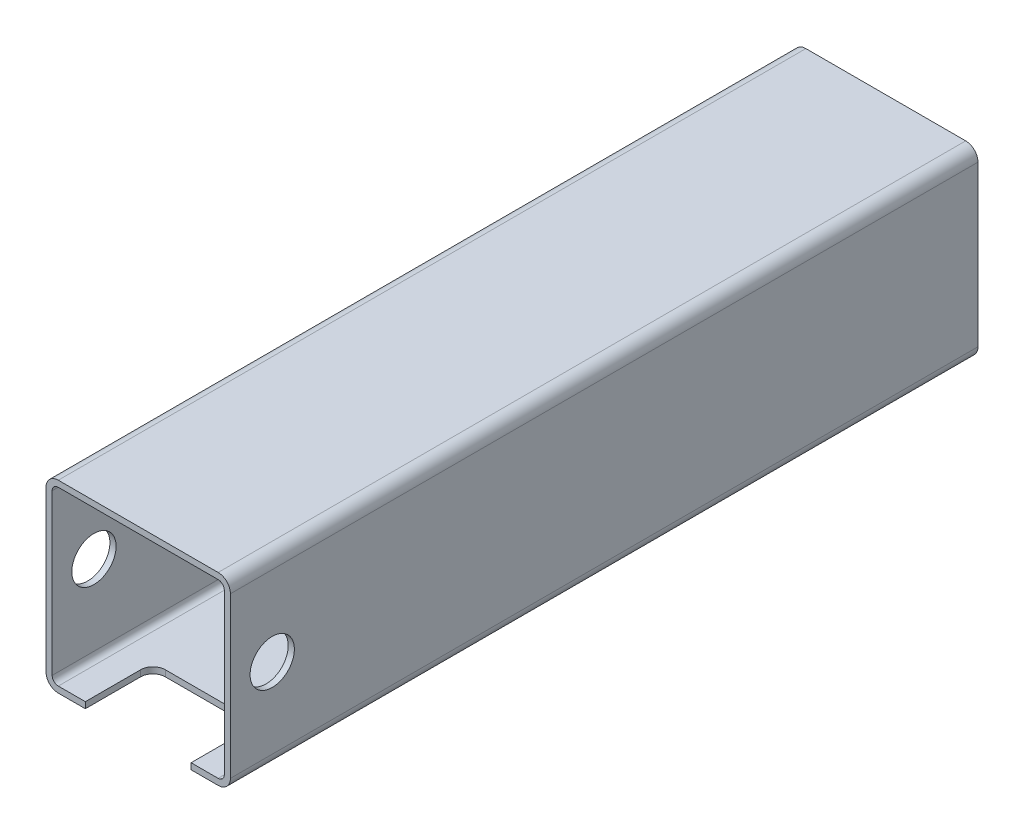
SolidWorks part; units mm, degrees
material "Q345"
ref_plane "Front Plane" through (0, 0, 0) normal (0, 0, 1) x (1, 0, 0)
ref_plane "Top Plane" through (0, 0, 0) normal (0, 1, 0) x (1, 0, 0)
ref_plane "Right Plane" through (0, 0, 0) normal (1, 0, 0) x (0, 0, -1)
sketch "Sketch1" plane through (0, 0, 0) normal (0, 0, 1) x (1, 0, 0)
  line L1 (0, 0) -> (150, 0)
  line L2 (0, 0) -> (0, 150)
  line L3 (0, 150) -> (150, 150)
  line L4 (150, 0) -> (150, 150)
  line L5 (5, 145) -> (145, 145)
  line L6 (5, 145) -> (5, 5)
  line L7 (5, 5) -> (145, 5)
  line L8 (145, 145) -> (145, 5)
  dimension "D1" = 150
  dimension "D2" = 150
  dimension "D3" = 5
  dimension "D4" = 5
  dimension "D5" = 5
  dimension "D6" = 5
extrude "Boss-Extrude1" add sketch "Sketch1" along normal blind 608
fillet "Fillet1" radius 10 4 edges at (150, 0, 304) (0, 0, 304) (0, 150, 304) (150, 150, 304)
fillet "Fillet2" radius 5 4 edges at (5, 5, 304) (145, 5, 304) (145, 145, 304) (5, 145, 304)
sketch "Sketch2" plane through (0, 0, 0) normal (-1, 0, 0) x (0, 0, 1)
  line L0 (0, 150) -> (608, 150) construction
  line L1 (608, 140) -> (608, 10) construction
  circle A0 centre (574, 75) radius 18
  dimension "D1" = 75
  dimension "D2" = 34
  dimension "D3" = 36
extrude "Cut-Extrude1" cut sketch "Sketch2" against normal through all
sketch "Sketch3" plane through (0, 0, 0) normal (0, -1, 0) x (1, 0, 0)
  line L0 (75, 608) -> (75, 0) construction
  line L1 (10, 608) -> (140, 608) construction
  line L2 (10, 0) -> (140, 0) construction
  line L4 (32, 608) -> (118, 608)
  line L5 (32, 608) -> (32, 553)
  line L6 (32, 553) -> (118, 553)
  line L7 (118, 608) -> (118, 553)
  dimension "D1" = 86
  dimension "D2" = 43
  dimension "D3" = 55
extrude "Cut-Extrude2" cut sketch "Sketch3" against normal blind 10
fillet "Fillet3" radius 10 2 edges at (118, 2.5, 553) (32, 2.5, 553)
